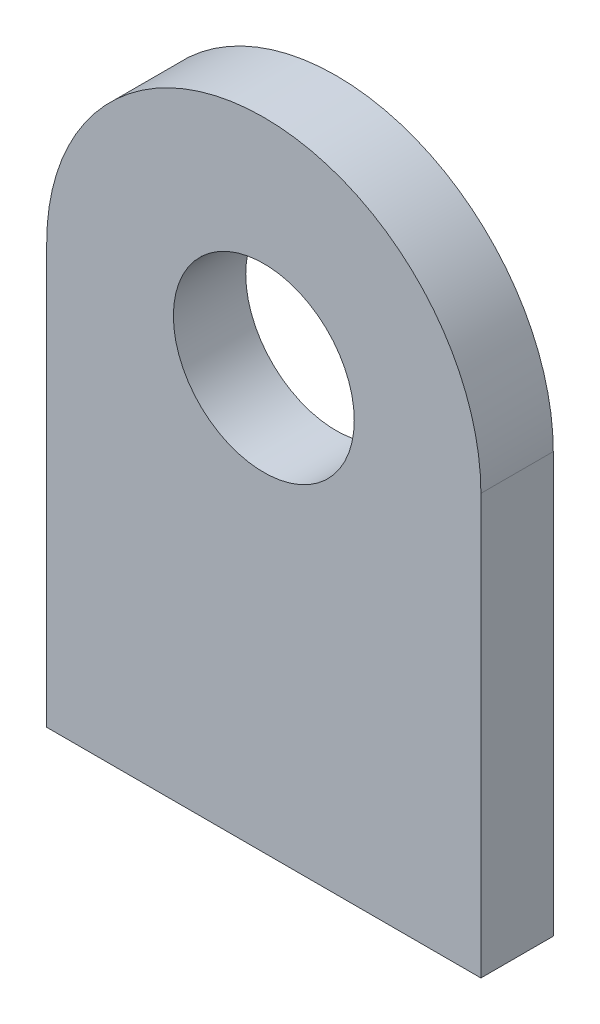
from build123d import *

# Parameters (mm, degrees)
SKETCH1_R           = 12.5
BOSS_EXTRUDE1_DEPTH = 10


with BuildPart() as part:
    # Sketch1 → Boss-Extrude1 (new body)
    with BuildSketch(Plane.XY):
        with BuildLine():
            Line((0, 0), (0, 58))
            ThreePointArc((0, 58), (30, 88), (60, 58))
            Line((60, 58), (60, 0))
            Line((60, 0), (0, 0))
        make_face()
        with Locations((30, 58)):
            Circle(SKETCH1_R, mode=Mode.SUBTRACT)
    extrude(amount=BOSS_EXTRUDE1_DEPTH)


solid = part.part
